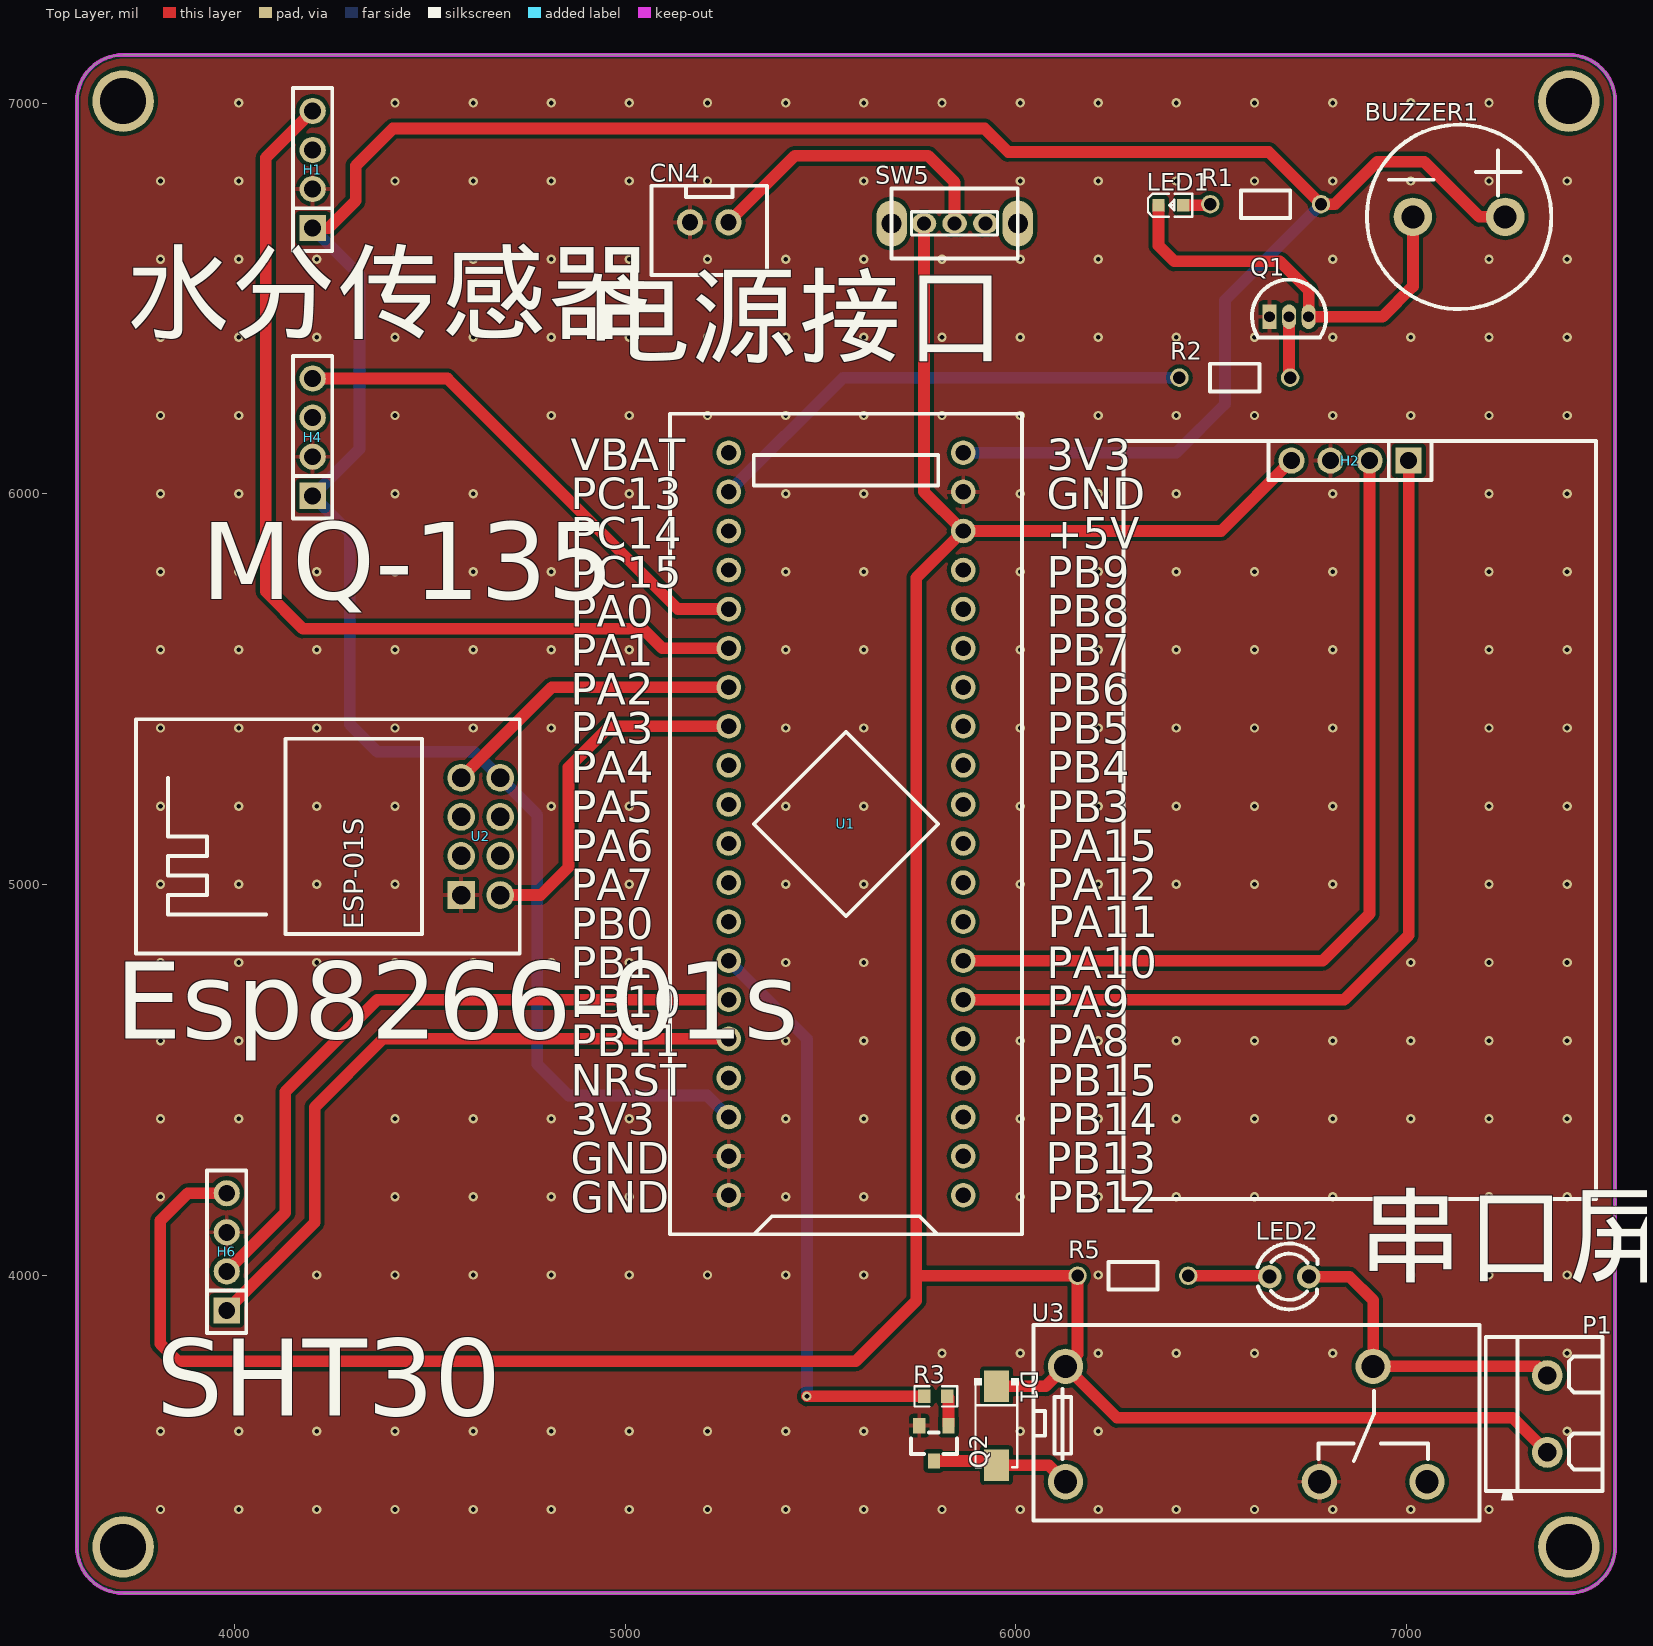
[diagram p0: Top Layer view]
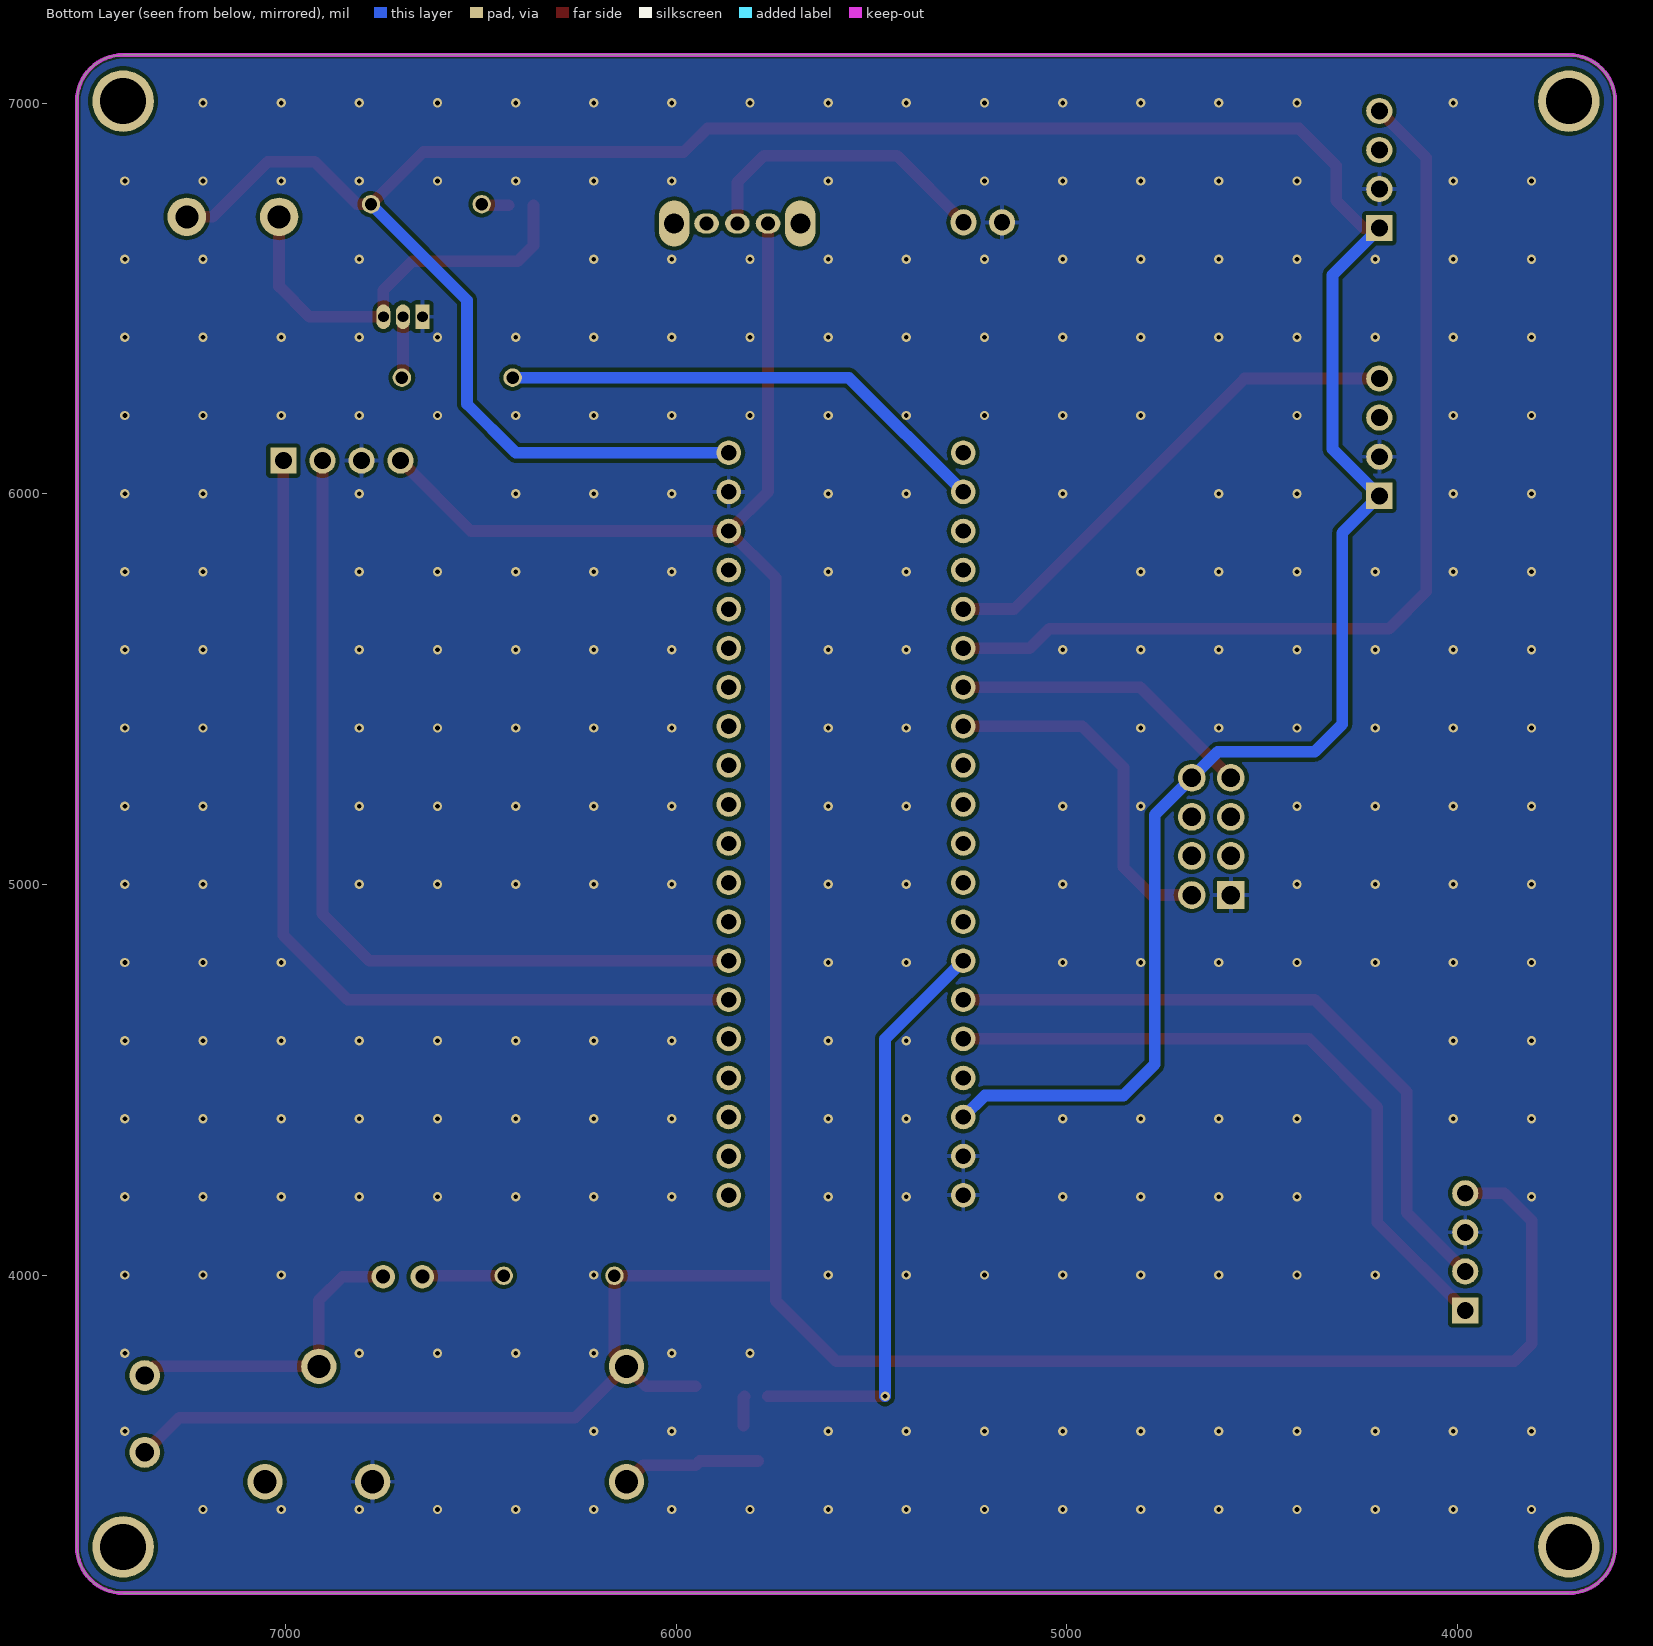
[diagram p1: Bottom Layer view, seen from below]
# Altium PCB MISC52093.pcbdoc
Units mil, origin at the board's own origin, x right, y up, seen from the top; angles counter-clockwise.
Board outline 3937.01 x 3937.01 mil, 2 copper layers (Top Layer, Bottom Layer), stack 62.206 mil thick; 20 components, 45 nets, 104 pads, 278 vias.

## Layer stack, top to bottom
Top Solder Mask Layer: solder mask 0.394, Dk 3.3
Top Layer: signal copper 1.379
Dielectric1: surface 59.449, FR4, Dk 4.5
Bottom Layer: signal copper 1.378
Bottom Solder Mask Layer: solder mask 0.394, Dk 3.3

## Board outline
3714.61,7123.5 ccw(c3714.61,7005.39) 3596.5,7005.39 3596.5,3304.61 ccw(c3714.61,3304.61) 3714.61,3186.5 7415.39,3186.5 ccw(c7415.39,3304.61) 7533.5,3304.61 7533.5,7005.39 ccw(c7415.39,7005.39) 7415.39,7123.5 3714.61,7123.5

## Design rules (kind name [scope] priority, off if disabled: settings)
BoardOutlineClearance copperThickness2oz_1 [All] p2 off: genericclearance=7.99 ignorepadtopadclearanceinfootprint=FALSE except(0: Arc-SplitContinuation Track-SplitContinuation SMDPad-SplitContinuation THPad-SplitContinuation Via-SplitContinuation Fill-SplitContinuation Region-SplitContinuation Poly-SplitContinuation Text-SplitContinuation Hole-SplitContinuation; 5.98: Arc-CutoutEdge Track-CutoutEdge SMDPad-CutoutEdge THPad-CutoutEdge Via-CutoutEdge Text-CutoutEdge; 6.9: Hole-OutlineEdge Hole-CutoutEdge; 10: Poly-OutlineEdge Poly-CutoutEdge; 11.81: Arc-OutlineEdge Track-OutlineEdge SMDPad-OutlineEdge THPad-OutlineEdge Via-OutlineEdge Fill-OutlineEdge Region-OutlineEdge Text-OutlineEdge Fill-CutoutEdge Region-CutoutEdge)
BoardOutlineClearance Plane_innerPlane_1 [All] p4 off: genericclearance=4.02 ignorepadtopadclearanceinfootprint=FALSE except(0: Arc-SplitContinuation Track-SplitContinuation SMDPad-SplitContinuation THPad-SplitContinuation Via-SplitContinuation Fill-SplitContinuation Region-SplitContinuation Poly-SplitContinuation Text-SplitContinuation Hole-SplitContinuation; 5.98: Arc-CutoutEdge Track-CutoutEdge SMDPad-CutoutEdge THPad-CutoutEdge Via-CutoutEdge Text-CutoutEdge; 6.9: Hole-OutlineEdge Hole-CutoutEdge; 10: Poly-OutlineEdge Poly-CutoutEdge; 11.81: Arc-OutlineEdge Track-OutlineEdge SMDPad-OutlineEdge THPad-OutlineEdge Via-OutlineEdge Fill-OutlineEdge Region-OutlineEdge Text-OutlineEdge Fill-CutoutEdge Region-CutoutEdge)
BoardOutlineClearance Copper_copperRegion_1 [All] p6 off: genericclearance=4.02 ignorepadtopadclearanceinfootprint=FALSE except(0: Arc-SplitContinuation Track-SplitContinuation SMDPad-SplitContinuation THPad-SplitContinuation Via-SplitContinuation Fill-SplitContinuation Region-SplitContinuation Poly-SplitContinuation Text-SplitContinuation Hole-SplitContinuation; 5.98: Arc-CutoutEdge Track-CutoutEdge SMDPad-CutoutEdge THPad-CutoutEdge Via-CutoutEdge Text-CutoutEdge; 6.9: Hole-OutlineEdge Hole-CutoutEdge; 10: Poly-OutlineEdge Poly-CutoutEdge; 11.81: Arc-OutlineEdge Track-OutlineEdge SMDPad-OutlineEdge THPad-OutlineEdge Via-OutlineEdge Fill-OutlineEdge Region-OutlineEdge Text-OutlineEdge Fill-CutoutEdge Region-CutoutEdge)
BoardOutlineClearance copperThickness1oz_1 [All] p8: genericclearance=4.02 ignorepadtopadclearanceinfootprint=FALSE except(0: Arc-SplitContinuation Track-SplitContinuation SMDPad-SplitContinuation THPad-SplitContinuation Via-SplitContinuation Fill-SplitContinuation Region-SplitContinuation Poly-SplitContinuation Text-SplitContinuation Hole-SplitContinuation; 5.98: Arc-CutoutEdge Track-CutoutEdge SMDPad-CutoutEdge THPad-CutoutEdge Via-CutoutEdge Text-CutoutEdge; 6.9: Hole-OutlineEdge Hole-CutoutEdge; 10: Poly-OutlineEdge Poly-CutoutEdge; 11.81: Arc-OutlineEdge Track-OutlineEdge SMDPad-OutlineEdge THPad-OutlineEdge Via-OutlineEdge Fill-OutlineEdge Region-OutlineEdge Text-OutlineEdge Fill-CutoutEdge Region-CutoutEdge)
Clearance copperThickness2oz [All] p1 off: gap=7.99 ignorepadtopadclearanceinfootprint=FALSE except(5.98: SMDPad-Track SMDPad-SMDPad THPad-Track SMDPad-THPad THPad-THPad Track-Via SMDPad-Via THPad-Via Via-Via Fill-SMDPad Region-SMDPad Fill-THPad Region-THPad Fill-Via Region-Via Fill-Fill Fill-Region Region-Region Arc-Track Arc-SMDPad Arc-THPad Arc-Via Fill-Arc Region-Arc Arc-Arc Text-Track SMDPad-Text Text-THPad Text-Via Fill-Text Region-Text Arc-Text Text-Text; 6.9: Hole-Track Hole-SMDPad Hole-THPad Hole-Via Fill-Hole Region-Hole Hole-Arc Hole-Text; 10: Poly-Track Poly-SMDPad Poly-THPad Poly-Via Poly-Fill Poly-Region Poly-Poly Poly-Arc Poly-Text Poly-Hole; 11.81: Fill-Track Region-Track)
Clearance Plane_innerPlane [All] p3 off: gap=4.02 ignorepadtopadclearanceinfootprint=FALSE except(5.98: SMDPad-Track SMDPad-SMDPad THPad-Track SMDPad-THPad THPad-THPad Track-Via SMDPad-Via THPad-Via Via-Via Fill-SMDPad Region-SMDPad Fill-THPad Region-THPad Fill-Via Region-Via Fill-Fill Fill-Region Region-Region Arc-Track Arc-SMDPad Arc-THPad Arc-Via Fill-Arc Region-Arc Arc-Arc Text-Track SMDPad-Text Text-THPad Text-Via Fill-Text Region-Text Arc-Text Text-Text; 6.9: Hole-Track Hole-SMDPad Hole-THPad Hole-Via Fill-Hole Region-Hole Hole-Arc Hole-Text; 10: Poly-Track Poly-SMDPad Poly-THPad Poly-Via Poly-Fill Poly-Region Poly-Poly Poly-Arc Poly-Text Poly-Hole; 11.81: Fill-Track Region-Track)
Clearance Copper_copperRegion [All] p5 off: gap=4.02 ignorepadtopadclearanceinfootprint=FALSE except(5.98: SMDPad-Track SMDPad-SMDPad THPad-Track SMDPad-THPad THPad-THPad Track-Via SMDPad-Via THPad-Via Via-Via Fill-SMDPad Region-SMDPad Fill-THPad Region-THPad Fill-Via Region-Via Fill-Fill Fill-Region Region-Region Arc-Track Arc-SMDPad Arc-THPad Arc-Via Fill-Arc Region-Arc Arc-Arc Text-Track SMDPad-Text Text-THPad Text-Via Fill-Text Region-Text Arc-Text Text-Text; 6.9: Hole-Track Hole-SMDPad Hole-THPad Hole-Via Fill-Hole Region-Hole Hole-Arc Hole-Text; 10: Poly-Track Poly-SMDPad Poly-THPad Poly-Via Poly-Fill Poly-Region Poly-Poly Poly-Arc Poly-Text Poly-Hole; 11.81: Fill-Track Region-Track)
Clearance copperThickness1oz [All] p7: gap=4.02 ignorepadtopadclearanceinfootprint=FALSE except(5.98: SMDPad-Track SMDPad-SMDPad THPad-Track SMDPad-THPad THPad-THPad Track-Via SMDPad-Via THPad-Via Via-Via Fill-SMDPad Region-SMDPad Fill-THPad Region-THPad Fill-Via Region-Via Fill-Fill Fill-Region Region-Region Arc-Track Arc-SMDPad Arc-THPad Arc-Via Fill-Arc Region-Arc Arc-Arc Text-Track SMDPad-Text Text-THPad Text-Via Fill-Text Region-Text Arc-Text Text-Text; 6.9: Hole-Track Hole-SMDPad Hole-THPad Hole-Via Fill-Hole Region-Hole Hole-Arc Hole-Text; 10: Poly-Track Poly-SMDPad Poly-THPad Poly-Via Poly-Fill Poly-Region Poly-Poly Poly-Arc Poly-Text Poly-Hole; 11.81: Fill-Track Region-Track)
DiffPairsRouting differentialPair [All] p1: maxlimit=6 minlimit=6 mostfreqgap=6 toplayer_minwidth=5 toplayer_prefwidth=10 toplayer_maxwidth=100 toplayer_mingap=6 toplayer_prefgap=6 toplayer_maxgap=6 bottomlayer_minwidth=5 bottomlayer_prefwidth=10 bottomlayer_maxwidth=100 bottomlayer_mingap=6 bottomlayer_prefgap=6 bottomlayer_maxgap=6 maxuncoupledlength=10
HoleToHoleClearance otherClearance [All] p1: gap=11.81 allowstackedmicrovias=TRUE
Length netLength [All] p1: minlimit=0 maxlimit=0
PasteMaskExpansion pasteMaskExpansion [All] p1: expansion=0
PlaneConnect innerPlane [All] p1: planeconnectstyle=Relief reliefexpansion=20 reliefentries=4 reliefconductorwidth=10 reliefairgap=10
PolygonConnect copperRegion [All] p1: connectstyle=Relief reliefconductorwidth=10 reliefentries=4 polygonreliefangle="90 Angle" airgapwidth=10 via.connectstyle=Relief via.reliefconductorwidth=10 via.reliefentries=4 via.polygonreliefangle="90 Angle" via.airgapwidth=10
RoutingVias viaSize [All] p1: holewidth=12.01 width=24.02 viastyle="Through Hole" minholewidth=11.81 minwidth=19.68 maxholewidth=248.03 maxwidth=393.7
SolderMaskExpansion solderMaskExpansion [IsVia] p1: expansion=-1000 istentingtop=TRUE
SolderMaskExpansion solderMaskExpansion [All] p2: expansion=2 istentingtop=FALSE
Width copperThickness2oz_2 [All] p1 off: maxlimit=100 minlimit=8 preferedwidth=10
Width copperThickness1oz_2 [All] p2: maxlimit=100 minlimit=5 preferedwidth=10

## Components (designator, comment, footprint, x,y, rotation, side; value= is the part's Value field where it differs from the comment)
BUZZER1 "buzzer" BUZ-TH_BD12.0-P6.00-D0.9-RD 7134.07,6708.93 r0 top
CN4 "XH2.54*2P_直插" CONN-TH_2P-P2.50-XH2.54-2P 5215,6695 r0 top
D1 "" SMA_1N4007 5950,3615 r270 top
H1 "" HDR-TH_4P-P2.54-V-F 4200,6830 r90 top
H2 "" HDR-TH_4P-P2.54-V-F 6855,6085 r180 top
H4 "" HDR-TH_4P-P2.54-V-F 4200,6145 r90 top
H6 "" HDR-TH_4P-P2.54-V-F 3980,4060 r90 top
LED1 "" LED_0603 6398.45,6738.93 r0 top
LED2 "" LED_TH-3mm 6699.47,3996.32 r0 top
P1 "KF301-2P接线端子" CONN-TH_XY301V-A-5.0-2P 7360,3645 r270 top
Q1 "" S8050_TO_92 6699.07,6453.34 r0 top
Q2 "" S8050_SOT-23 5790,3570 r90 top
R1 "220Ω" Res_1/8W 6639.09,6738.93 r0 top
R2 "10kΩ" Res_1/8W 6560,6295 r0 top
R3 "1K" R0603 5795,3690 r0 top
R5 "1kΩ" Res_1/8W 6299.47,3996.32 r0 top
SW5 "" 拨动开关 5837.9,6692.05 r0 top
U1 "STM32F103C8T6-Card" CONN-TH_L53.3-W22.9_STM32F103C8T6-CARD 5565,5155 r90 top
U2 "ESP-01S" WIFIM-TH_ESP-01S 4630,5123.21 r90 top
U3 "SSKD6132" RELAY-TH_G2R-1 6589.47,3619.17 r0 top

## Footprints (in the part's own frame and the unit in brackets; to place one, negate y for a bottom-side part, rotate by r counter-clockwise, add the part's x,y. Pads: shape width x height; smd on the part's side, far side on the other; paste and mask are expansions set on the pad)
BUZ-TH_BD12.0-P6.00-D0.9-RD [mm]
  round 2.5 hole 1.5 paste+0 mask+0.05: 1(-3,0) 2(3,0)
  silkscreen extent -5.99,-5.99 5.99,5.99
CONN-TH_2P-P2.50-XH2.54-2P [mm]
  round 1.7 hole 1.05 paste+0 mask+0.05: 1(1.25,0) 2(-1.25,0)
  silkscreen extent -3.75,-3.42 3.75,2.37
CONN-TH_L53.3-W22.9_STM32F103C8T6-CARD [mm]
  round 1.6 hole 1: 1(-24.13,-7.62) 2(-21.59,-7.62) 3(-19.05,-7.62) 4(-16.51,-7.62) 5(-13.97,-7.62) 6(-11.43,-7.62) 7(-8.89,-7.62) 8(-6.35,-7.62) 9(-3.81,-7.62) 10(-1.27,-7.62) 11(1.27,-7.62) 12(3.81,-7.62) 13(6.35,-7.62) 14(8.89,-7.62) 15(11.43,-7.62) 16(13.97,-7.62) 17(16.51,-7.62) 18(19.05,-7.62) 19(21.59,-7.62) 20(24.13,-7.62) 21(24.13,7.62) 22(21.59,7.62) 23(19.05,7.62) 24(16.51,7.62) 25(13.97,7.62) 26(11.43,7.62) 27(8.89,7.62) 28(6.35,7.62) 29(3.81,7.62) 30(1.27,7.62) 31(-1.27,7.62) 32(-3.81,7.62) 33(-6.35,7.62) 34(-8.89,7.62) 35(-11.43,7.62) 36(-13.97,7.62) 37(-16.51,7.62) 38(-19.05,7.62) 39(-21.59,7.62) 40(-24.13,7.62)
  silkscreen extent -26.67,-11.43 26.67,11.43
CONN-TH_XY301V-A-5.0-2P [mm]
  round 2 hole 1.2: 1(-2.5,0) 2(2.5,0)
  silkscreen extent -5,-4 5.6,3.6
HDR-TH_4P-P2.54-V-F [mm]
  rect 1.7x1.7 hole 1.1: 1(-3.81,0)
  round 1.7 hole 1.1: 2(-1.27,0) 3(1.27,0) 4(3.81,0)
  silkscreen extent -5.29,-1.27 5.29,1.27
LED_0603 [mil]
  rect 31.5x31.5 smd paste+0 mask+2: 1(-33.5,-0.4) 2(29.5,-0.2)
  silkscreen extent -61,-30 53,30
LED_TH-3mm [mil]
  round 60 hole 36 paste+0 mask+2: 1(-50,0) 2(50,0)
  silkscreen extent -81,-84 72,85
R0603 [mil]
  rect 31.75x34.02 smd paste-3937.01 mask+2: 1(-29.66,0) 2(29.66,0)
  silkscreen extent -55,-26 55,26
RELAY-TH_G2R-1 [mm]
  round 2.3 hole 1.5: 1(-11.75,-3.75) 2(4.75,-3.75) 3(11.75,-3.75) 4(8.25,3.75) 5(-11.75,3.75)
  silkscreen extent -13.83,-6.26 15.17,6.44
Res_1/8W [mil]
  round 47.2 hole 31.5 paste+0 mask+2: 1(-141.7,2.48) 2(141.7,2.48)
  silkscreen extent -63,-33 63,38
S8050_SOT-23 [mm]
  rect 1x0.8 smd paste+0 mask+0.051: 1(1.15,-0.95) 2(1.15,0.95) 3(-1.15,0)
  silkscreen extent -0.7,-1.5 0.7,1.5
S8050_TO_92 [mil]
  rect 35.4x63 hole 27.6 paste+0 mask+2: 1(-50,0)
  oval 35.4x63 hole 27.6 paste+0 mask+2: 2(0,0) 3(50,0)
  silkscreen extent -95,-53 95,95
SMA_1N4007 [mil]
  rect 80.57x63.78 smd paste+0 mask+2: 1(-101,0) 2(101,0)
  silkscreen extent -121,-57 106,57
WIFIM-TH_ESP-01S [mm]
  rect 1.8x1.8 hole 1.2: 1(-3.81,1.27)
  round 1.8 hole 1.2: 2(-1.27,1.27) 3(1.27,1.27) 4(3.81,1.27) 5(3.81,-1.27) 6(1.27,-1.27) 7(-1.27,-1.27) 8(-3.81,-1.27)
  silkscreen extent -7.62,-2.54 7.62,22.4
拨动开关 [mil]
  oval 63x51.2 hole 35.4 paste+0 mask+2: 1(-73.4,0) 2(5,0) 3(84,0)
  oval 78.7x118.1 hole 51.2 paste+0 mask+2: 4(166.7,0) 5(-156.1,0)
  silkscreen extent -156,-90 167,90

## Free pads (board coordinates)
  round 157.48 hole 118.11: 1(3714.61,7005.39) 1(3714.61,3304.61) 1(7415.39,7005.39) 1(7415.39,3304.61)

## Via types
v1: diameter 24.02, hole 12, Top Layer to Bottom Layer, 278 vias

## Nets (pads, with @x,y where several pads share a name; then routed paths per layer and width w, separated by ;. In a path a pad name is that pad's centre, name@x,y a point inside that pad or via, vN(x,y) a via of type N, cw(c..) or ccw(c..) an arc to the next point about the centre after c; other vN are vias at no path point)
$1N17118: CN4.1 SW5.2 | length 782.3
  Top Layer w30: CN4.1 5434.22,6865 5775,6865 5842.9,6797.1 SW5.2
$1N17197: LED2.1 R5.2 | length 209.3
  Top Layer w30: R5.2 6647,3998.79 LED2.1
$1N17198: LED2.2 P1.1 U3.4 | length 814.2
  Top Layer w30: LED2.2 6853.68,3996.32 6914.27,3935.73 U3.4 7336.61,3766.82 P1.1
$1N17201: Q2.1 R3.2 | length 75.9
  Top Layer w30: R3.2 5827.4,3687.26 Q2.1
$1N17202: D1.2 Q2.3 U3.1 | length 358.9
  Top Layer w30: Q2.3 5939.28,3524.72 D1.2 6084.39,3514 U3.1
$1N17204: Q1.2 R2.2 | length 157
  Top Layer w30: Q1.2 6699.07,6300.11 R2.2
$1N17206: BUZZER1.1 LED1.1 Q1.3 | length 1079.5
  Top Layer w30: LED1.1 6364.95,6635.05 6405,6595 6675,6595 6749.07,6520.93 Q1.3 6938.34,6453.34 7015.96,6530.96 BUZZER1.1
$1N17209: LED1.2 R1.1 | length 70.5
  Top Layer w30: LED1.2 6494.71,6738.73 R1.1
+5V: D1.1 H2.4 H6.4 P1.2 R5.1 SW5.1 U1.18 U3.5 | length 8474.6
  Top Layer w30: H6.4 3880,4210 3810,4140 3810,3825 3855,3780 5590,3780 5745,3935 5745,3998.87 ; SW5.1 5764.5,6005.5 U1.18 ; D1.1 6076.06,3716 U3.5 ; H2.4 6525,5905 U1.18 ; P1.2 7271.57,3635 6258.69,3635 U3.5 ; 5745,3998.87 5745.07,3998.79 R5.1 6157.77,3797.72 U3.5 ; 5745,3998.87 5745,5785 U1.18
GND: CN4.2 H1.2 H2.3 H4.2 H6.3 Q1.1 Q2.2 U1.19 U1.39 U1.40 U2.1 U3.2
  other v1: 3810.6,3400.6 4010.6,3400.6 4210.6,3400.6 4410.6,3400.6 4610.6,3400.6 4810.6,3400.6 5010.6,3400.6 5210.6,3400.6 5410.6,3400.6 5610.6,3400.6 5810.6,3400.6 6010.6,3400.6 6210.6,3400.6 6410.6,3400.6 6610.6,3400.6 6810.6,3400.6 7010.6,3400.6 7210.6,3400.6 3810.6,3600.6 4010.6,3600.6 4210.6,3600.6 4410.6,3600.6 4610.6,3600.6 4810.6,3600.6 5010.6,3600.6 5210.6,3600.6 5410.6,3600.6 5610.6,3600.6 6010.6,3600.6 6210.6,3600.6 7410.6,3600.6 5810.6,3800.6 6010.6,3800.6 6210.6,3800.6 6410.6,3800.6 6610.6,3800.6 6810.6,3800.6 7410.6,3800.6 4210.6,4000.6 4410.6,4000.6 4610.6,4000.6 4810.6,4000.6 5010.6,4000.6 5210.6,4000.6 5410.6,4000.6 5610.6,4000.6 6210.6,4000.6 7010.6,4000.6 7210.6,4000.6 7410.6,4000.6 3810.6,4200.6 4410.6,4200.6 4610.6,4200.6 4810.6,4200.6 5010.6,4200.6 5410.6,4200.6 5610.6,4200.6 6010.6,4200.6 6210.6,4200.6 6410.6,4200.6 6610.6,4200.6 6810.6,4200.6 7010.6,4200.6 7210.6,4200.6 7410.6,4200.6 3810.6,4400.6 4010.6,4400.6 4410.6,4400.6 4610.6,4400.6 4810.6,4400.6 5010.6,4400.6 5410.6,4400.6 5610.6,4400.6 6010.6,4400.6 6210.6,4400.6 6410.6,4400.6 6610.6,4400.6 6810.6,4400.6 7010.6,4400.6 7210.6,4400.6 7410.6,4400.6 3810.6,4600.6 4010.6,4600.6 5410.6,4600.6 5610.6,4600.6 6010.6,4600.6 6210.6,4600.6 6410.6,4600.6 6610.6,4600.6 6810.6,4600.6 7010.6,4600.6 7210.6,4600.6 7410.6,4600.6 3810.6,4800.6 4010.6,4800.6 4210.6,4800.6 4410.6,4800.6 4610.6,4800.6 4810.6,4800.6 5010.6,4800.6 5410.6,4800.6 5610.6,4800.6 7010.6,4800.6 7210.6,4800.6 7410.6,4800.6 3810.6,5000.6 4010.6,5000.6 4210.6,5000.6 4410.6,5000.6 5010.6,5000.6 5410.6,5000.6 5610.6,5000.6 6010.6,5000.6 6210.6,5000.6 6410.6,5000.6 6610.6,5000.6 6810.6,5000.6 7210.6,5000.6 7410.6,5000.6 3810.6,5200.6 4010.6,5200.6 4210.6,5200.6 4410.6,5200.6 4810.6,5200.6 5010.6,5200.6 5410.6,5200.6 5610.6,5200.6 6010.6,5200.6 6210.6,5200.6 6410.6,5200.6 6610.6,5200.6 6810.6,5200.6 7210.6,5200.6 7410.6,5200.6 3810.6,5400.6 4010.6,5400.6 4210.6,5400.6 4410.6,5400.6 4610.6,5400.6 4810.6,5400.6 5410.6,5400.6 5610.6,5400.6 6010.6,5400.6 6210.6,5400.6 6410.6,5400.6 6610.6,5400.6 6810.6,5400.6 7210.6,5400.6 7410.6,5400.6 3810.6,5600.6 4010.6,5600.6 4210.6,5600.6 4410.6,5600.6 4610.6,5600.6 4810.6,5600.6 5010.6,5600.6 5410.6,5600.6 5610.6,5600.6 6010.6,5600.6 6210.6,5600.6 6410.6,5600.6 6610.6,5600.6 6810.6,5600.6 7210.6,5600.6 7410.6,5600.6 3810.6,5800.6 4010.6,5800.6 4210.6,5800.6 4410.6,5800.6 4610.6,5800.6 4810.6,5800.6 5410.6,5800.6 5610.6,5800.6 6010.6,5800.6 6210.6,5800.6 6410.6,5800.6 6610.6,5800.6 6810.6,5800.6 7210.6,5800.6 7410.6,5800.6 3810.6,6000.6 4010.6,6000.6 4410.6,6000.6 4610.6,6000.6 5010.6,6000.6 5410.6,6000.6 5610.6,6000.6 6010.6,6000.6 6210.6,6000.6 6410.6,6000.6 6810.6,6000.6 7210.6,6000.6 7410.6,6000.6 3810.6,6200.6 4010.6,6200.6 4410.6,6200.6 4810.6,6200.6 5010.6,6200.6 5210.6,6200.6 5410.6,6200.6 5610.6,6200.6 5810.6,6200.6 6010.6,6200.6 6210.6,6200.6 6410.6,6200.6 6610.6,6200.6 6810.6,6200.6 7010.6,6200.6 7210.6,6200.6 7410.6,6200.6 3810.6,6400.6 4010.6,6400.6 4210.6,6400.6 4410.6,6400.6 4610.6,6400.6 4810.6,6400.6 5010.6,6400.6 5210.6,6400.6 5410.6,6400.6 5610.6,6400.6 5810.6,6400.6 6010.6,6400.6 6210.6,6400.6 6410.6,6400.6 6610.6,6400.6 6810.6,6400.6 7010.6,6400.6 7210.6,6400.6 7410.6,6400.6 3810.6,6600.6 4010.6,6600.6 4210.6,6600.6 4410.6,6600.6 4610.6,6600.6 4810.6,6600.6 5010.6,6600.6 5210.6,6600.6 5410.6,6600.6 5610.6,6600.6 5810.6,6600.6 6010.6,6600.6 6210.6,6600.6 6810.6,6600.6 7210.6,6600.6 7410.6,6600.6 3810.6,6800.6 4010.6,6800.6 4410.6,6800.6 4610.6,6800.6 4810.6,6800.6 5010.6,6800.6 5210.6,6800.6 5610.6,6800.6 6010.6,6800.6 6210.6,6800.6 6410.6,6800.6 6610.6,6800.6 6810.6,6800.6 7010.6,6800.6 7210.6,6800.6 7410.6,6800.6 4010.6,7000.6 4410.6,7000.6 4610.6,7000.6 4810.6,7000.6 5010.6,7000.6 5210.6,7000.6 5410.6,7000.6 5610.6,7000.6 5810.6,7000.6 6010.6,7000.6 6210.6,7000.6 6410.6,7000.6 6610.6,7000.6 6810.6,7000.6 7010.6,7000.6 7210.6,7000.6
NRST: U1.37
PA0: H4.4 U1.25 | length 1309.4
  Top Layer w30: H4.4 4545,6295 5135,5705 U1.25
PA1: H1.4 U1.26 | length 2524.8
  Top Layer w30: H1.4 4080,6860 4080,5750 4175,5655 5045,5655 5095,5605 U1.26
PA2: U1.27 U2.4 | length 781
  Top Layer w30: U2.4 4811.79,5505 U1.27
PA3: U1.28 U2.8 | length 913.2
  Top Layer w30: U2.8 4783.21,4973.21 4855,5045 4855,5300 4960,5405 U1.28
PA4: U1.29
PA5: U1.30
PA6: U1.31
PA7: U1.32
PA8: U1.5
PA9: H2.1 U1.6 | length 2423.3
  Top Layer w30: U1.6 6840,4705 7005,4870 H2.1
PA10: H2.2 U1.7 | length 2249.7
  Top Layer w30: U1.7 6785,4805 6905,4925 H2.2
PA11: U1.8
PA12: U1.9
PA15: U1.10
PB0: U1.33
PB1: R3.1 U1.34 | length 1498.2
  Top Layer w30: v1(5465,3690) R3.1
  Bottom Layer w30: U1.34 5465,4605 v1(5465,3690)
PB3: U1.11
PB4: U1.12
PB5: U1.13
PB6: U1.14
PB7: U1.15
PB8: U1.16
PB9: U1.17
PB10: H6.2 U1.35 | length 1754.5
  Top Layer w30: H6.2 4130,4160 4130,4470 4365,4705 U1.35
PB11: H6.1 U1.36 | length 1745.7
  Top Layer w30: H6.1 4205,4135 4205,4430 4380,4605 U1.36
PB12: U1.1
PB13: U1.2
PB14: U1.3
PB15: U1.4
PC13: R2.1 U1.22 | length 1274.4
  Bottom Layer w30: U1.22 5557.47,6297.48 R2.1
PC14: U1.23
PC15: U1.24
VBAT: U1.21
VCC: BUZZER1.2 H1.1 H4.1 R1.2 U1.20 U1.38 U2.5 | length 7898
  Top Layer w30: H1.1 4240,6680 4310,6750 4310,6840 4405,6935 5920,6935 5980,6875 6647.2,6875 R1.2 6816.41,6741.41 6925,6850 7045,6850 7186.07,6708.93 BUZZER1.2
  Bottom Layer w30: H1.1 4320,6560 4320,6115 H4.1 4295,5900 4295,5410 4365,5340 4613.21,5340 U2.5 4775,5178.21 4775,4540 4855,4460 5210,4460 U1.38 ; U1.20 6410,6105 6535,6230 6535,6495.63 R1.2
pads on no net: H1.3 H4.3 SW5.3 SW5.4 SW5.5 U2.2 U2.3 U2.6 U2.7 U3.3

## Polygon pours and split planes (outlines as drawn)
GND on Bottom Layer (solid, remove dead copper, pour order 2): 3525,7245 3525,3080 7700,3080 7700,7245
GND on Top Layer (solid, remove dead copper, pour order 2): 3000,7415 3000,3000 7930,3000 7930,7415

## Keep-outs
Board Outline Layer:
  the board outline again, w10

## Silkscreen, mask and mechanical layers (free items; w line width, h text height)
Top Silkscreen Layer:
  lines w10: 6275,4195 6275,6135 7485,6135 7485,4195 6275,4195
  text "水分传感器" at 3720,6420 h196.85
  text "电源接口" at 4900,6360 h196.85
  text "VBAT" at 4860.95,6060 h80
  text "3V3" at 6079.16,6060 h80
  text "PC13" at 4860.95,5960 h80
  text "GND" at 6079.16,5960 h80
  text "PC14" at 4860.95,5860 h80
  text "+5V" at 6079.16,5860 h80
  text "PC15" at 4860.95,5760 h80
  text "PB9" at 6079.16,5760 h80
  text "MQ-135" at 3915,5730 h196.85
  text "PA0" at 4860.95,5660 h80
  text "PB8" at 6079.16,5660 h80
  text "PA1" at 4860.95,5560 h80
  text "PB7" at 6079.16,5560 h80
  text "PA2" at 4860.95,5460 h80
  text "PB6" at 6079.16,5460 h80
  text "PA3" at 4860.95,5360 h80
  text "PB5" at 6079.16,5360 h80
  text "PA4" at 4860.95,5260 h80
  text "PB4" at 6079.16,5260 h80
  text "PA5" at 4860.95,5160 h80
  text "PB3" at 6079.16,5160 h80
  text "PA6" at 4860.95,5060 h80
  text "PA15" at 6079.16,5060 h80
  text "PA7" at 4860.95,4960 h80
  text "PA12" at 6079.16,4960 h80
  text "PA11" at 6080.95,4865 h80
  text "PB0" at 4860.95,4860 h80
  text "PB1" at 4860.95,4760 h80
  text "PA10" at 6079.16,4760 h80
  text "PB10" at 4860.95,4660 h80
  text "PA9" at 6079.16,4660 h80
  text "Esp8266-01s" at 3695,4605 h196.85
  text "PB11" at 4860.95,4560 h80
  text "PA8" at 6079.16,4560 h80
  text "NRST" at 4860.95,4460 h80
  text "PB15" at 6079.16,4460 h80
  text "3V3" at 4860.95,4360 h80
  text "PB14" at 6079.16,4360 h80
  text "GND" at 4860.95,4260 h80
  text "PB13" at 6075.95,4260 h80
  text "GND" at 4860.95,4160 h80
  text "PB12" at 6079.16,4160 h80
  text "串口屏" at 6875,4005 h196.85
  text "SHT30" at 3800,3640 h196.85